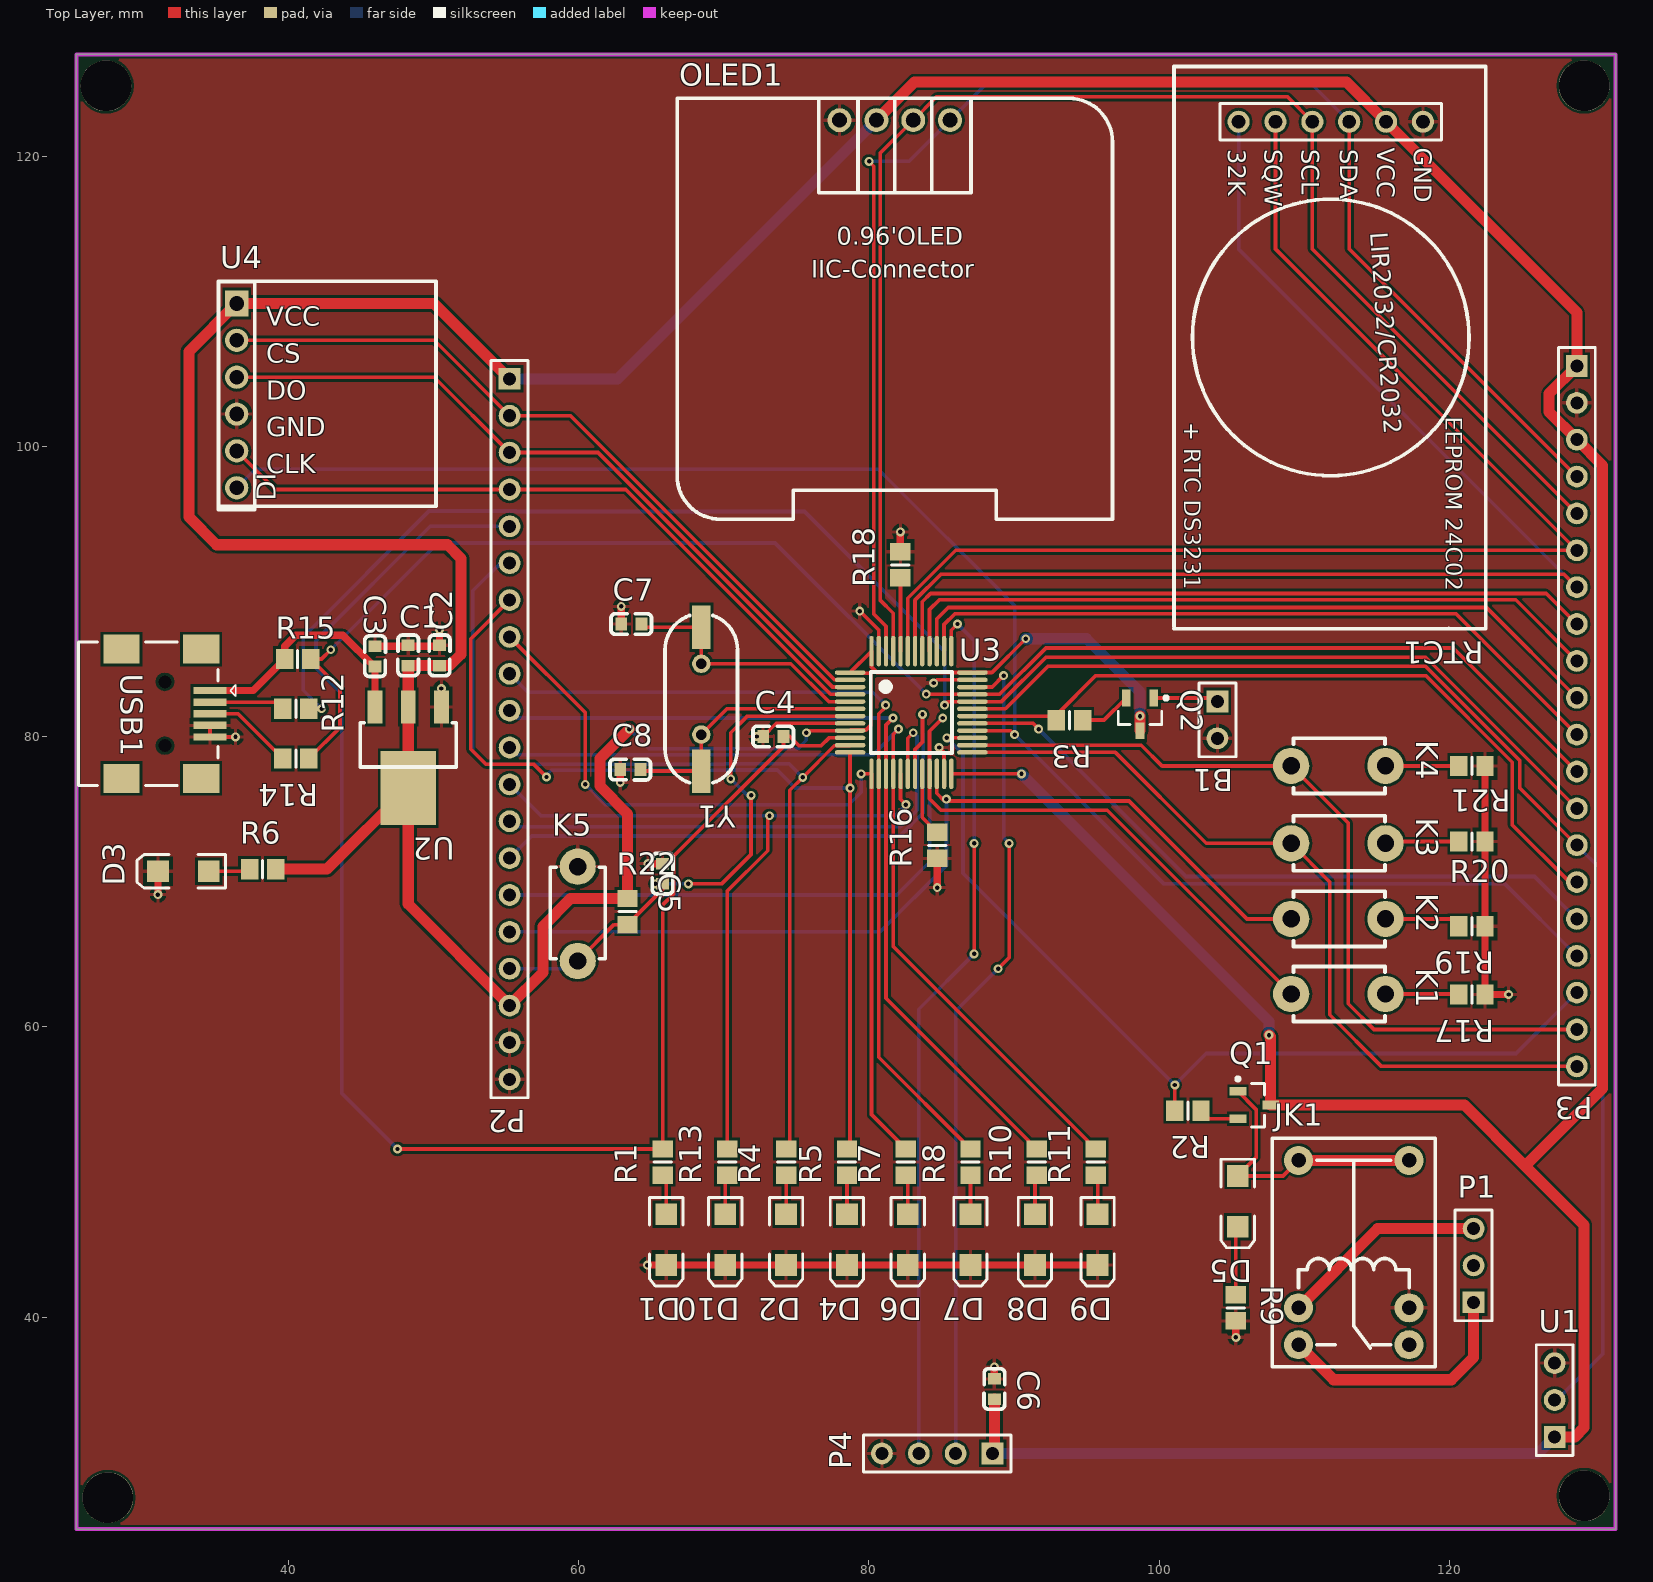
[diagram p0: Top Layer view]
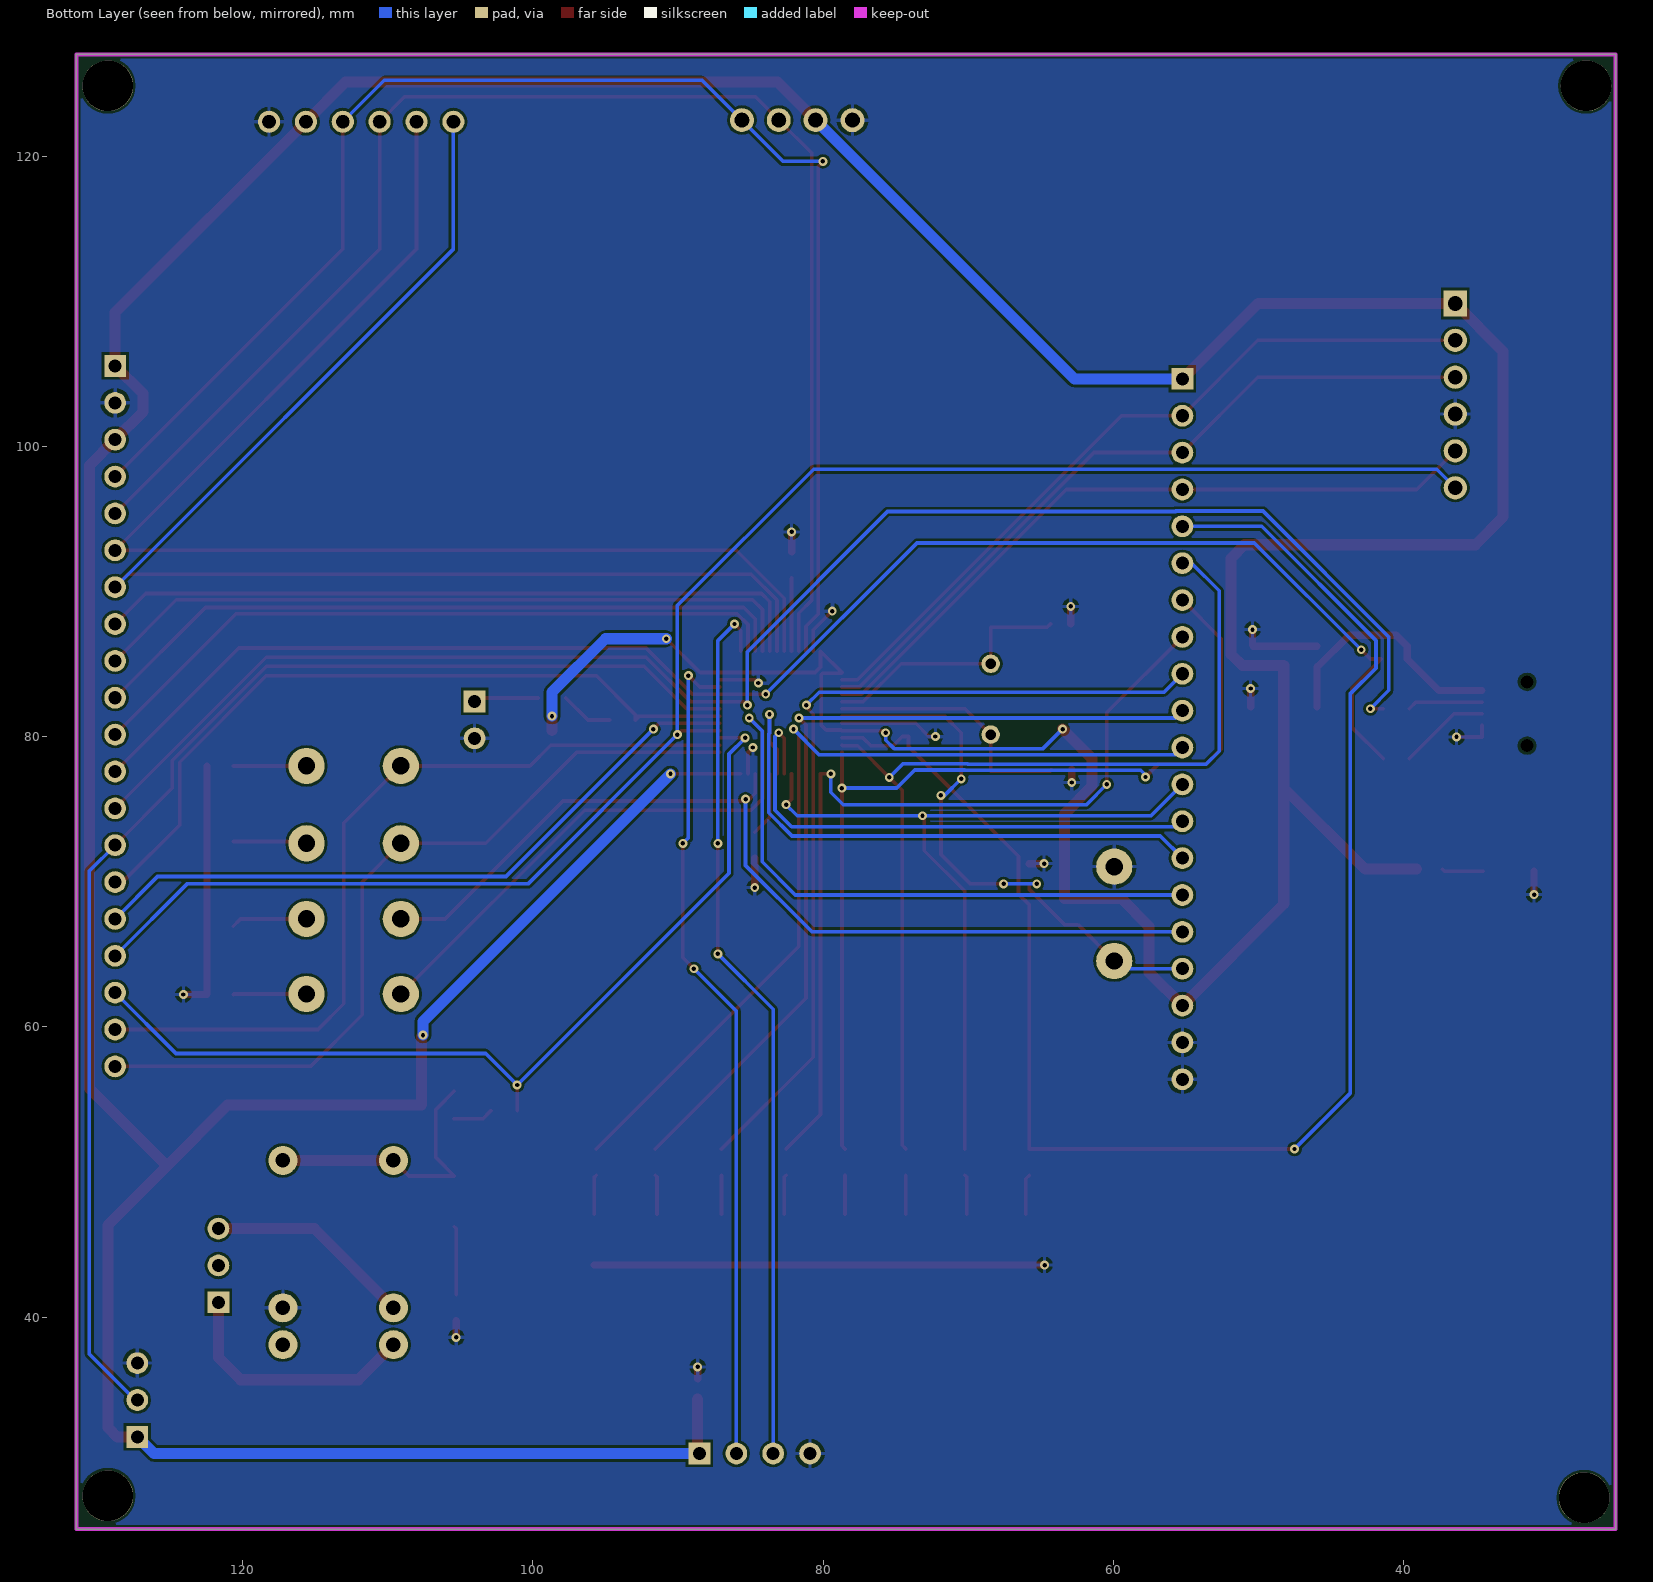
[diagram p1: Bottom Layer view, seen from below]
# Altium PCB MISC82098.PcbDoc
Units mm, origin at the board's own origin, x right, y up, seen from the top; angles counter-clockwise.
Board outline 106.05 x 101.6 mm, 2 copper layers (Top Layer, Bottom Layer); 61 components, 64 nets, 241 pads, 57 vias.

## Layer stack, top to bottom (the 12.6 mil dielectric is the usual default, probably not edited)
Top Solder: solder mask 0.0102, Solder Resist, Dk 3.5
Top Layer: signal copper 0.0356
Dielectric 1: dielectric 0.32, FR-4, Dk 4.8
Bottom Layer: signal copper 0.0356
Bottom Solder: solder mask 0.0102, Solder Resist, Dk 3.5

## Board outline
25.4,25.4 25.4,127 131.445,127 131.445,25.4

## Design rules (kind name [scope] priority, off if disabled: settings)
Clearance [All] p1: gap=0.178
MinimumSolderMaskSliver [All] p1: minsoldermaskwidth=0
PolygonConnect [All] p1: connectstyle=Relief reliefconductorwidth=0.254 reliefentries=4 polygonreliefangle="90 Angle" airgapwidth=0.254
RoutingVias [All] p1: holewidth=0.711 width=1.27 viastyle="Through Hole" minholewidth=0.711 minwidth=1.27 maxholewidth=0.711 maxwidth=1.27
SilkToSilkClearance [All] p1: silktosilkclearance=0
SilkToSolderMaskClearance [IsPad] p1: minsilkscreentomaskgap=0 clearancetoexposedcopper=TRUE
SolderMaskExpansion [All] p1: expansion=0.102
Width [All] p1: maxlimit=0.762 minlimit=0.254 preferedwidth=0.254
27 further rules are at their usual default settings.

## Components (designator, comment, footprint, x,y, rotation, side; value= is the part's Value field where it differs from the comment)
B1 "BEEP" HDR1X2 104.013,82.423 r270 top
C1 "10uF" C0603 48.26,85.598 r270 top
C2 "0.1uF" C0603 50.419,85.598 r270 top
C3 "10uF" C0603 45.977,85.541 r270 top
C4 "0.1uF" C0603 73.406,80.01 r0 top
C5 "0.1uF" C0603 65.789,70.558 r270 top
C6 "100NF" C0603 88.646,35.052 r270 top
C7 "20pF" C0603 63.627,87.757 r0 top
C8 "20pF" C0603 63.557,77.727 r0 top
D1 "POWER" 3.2X1.6X1.1 66.04,45.339 r270 top
D2 "POWER" 3.2X1.6X1.1 74.295,45.339 r270 top
D3 "POWER" 3.2X1.6X1.1 32.764,70.719 r180 top
D4 "POWER" 3.2X1.6X1.1 78.486,45.339 r270 top
D5 "POWER" 3.2X1.6X1.1 105.41,47.978 r270 top
D6 "POWER" 3.2X1.6X1.1 82.677,45.339 r270 top
D7 "POWER" 3.2X1.6X1.1 86.995,45.339 r270 top
D8 "POWER" 3.2X1.6X1.1 91.44,45.339 r270 top
D9 "POWER" 3.2X1.6X1.1 95.758,45.339 r270 top
D10 "POWER" 3.2X1.6X1.1 70.104,45.339 r270 top
JK1 "HK4100F-DC5V-SHG" HK4100F 113.411,44.45 r90 top
K1 "KEY" DIP-3X6X4.3 109.093,62.265 r0 top
K2 "KEY" DIP-3X6X4.3 109.093,67.437 r0 top
K3 "KEY" DIP-3X6X4.3 109.093,72.649 r0 top
K4 "KEY" DIP-3X6X4.3 109.093,77.978 r0 top
K5 "KEY" DIP-3X6X4.3 59.939,64.538 r90 top
OLED1 "0.96OLED_4P_MODULE_JX" 0.96OLED_4P 81.788,109.474 r0 top
P1 "Header 3" HDR1X3 121.666,41.021 r90 top
P2 "Header 20" HDR1X20 55.245,104.648 r270 top
P3 "Header 20" HDR1X20 128.778,105.537 r270 top
P4 "Header 4" HDR1X4 88.519,30.607 r180 top
Q1 "PNP" SOT-23B_N 106.553,54.61 r0 top
Q2 "PNP" SOT-23B_N 98.679,81.534 r270 top
R1 "330" 6-0805_N 65.786,50.684 r90 top
R2 "1K" 6-0805_N 101.981,54.229 r180 top
R3 "4.7K" 6-0805_N 93.822,81.137 r180 top
R4 "330" 6-0805_N 74.295,50.684 r90 top
R5 "330" 6-0805_N 78.486,50.684 r90 top
R6 "330" 6-0805_N 38.227,70.866 r0 top
R7 "330" 6-0805_N 82.55,50.684 r90 top
R8 "330" 6-0805_N 86.995,50.684 r90 top
R9 "1K" 6-0805_N 105.283,40.64 r270 top
R10 "330" 6-0805_N 91.567,50.684 r90 top
R11 "330" 6-0805_N 95.631,50.684 r90 top
R12 "100" 6-0805_N 40.513,81.915 r180 top
R13 "330" 6-0805_N 70.231,50.684 r90 top
R14 "100" 6-0805_N 40.513,78.486 r180 top
R15 "10K" 6-0805_N 40.64,85.344 r180 top
R16 "10K" 6-0805_N 84.709,72.506 r90 top
R17 "10K" 6-0805_N 121.55,62.23 r180 top
R18 "10K" 6-0805_N 82.169,91.832 r90 top
R19 "10K" 6-0805_N 121.55,66.929 r180 top
R20 "10K" 6-0805_N 121.55,72.771 r180 top
R21 "10K" 6-0805_N 121.55,77.978 r180 top
R22 "10K" 6-0805_N 63.373,67.945 r90 top
RTC1 "DS3231-RTC-SINGLE-HEADER" DS3231-RTC-24C32-EEPROM-SINGLE-HEADER 111.76,106.807 r270 top
U1 "DHT11" HDR1X3 127.254,31.75 r90 top
U2 "AMS1117" SOT223 48.26,82.042 r180 top
U3 "STM32F103C8T6" "LQFP48 7X7" 82.931,81.661 r270 top
U4 "W25Q128  SPI-Flash外部存储器" "SPI FLASH" 42.672,103.505 r0 top
USB1 "MINI-USB" USB-MINI-A 34.604,83.175 r270 top
Y1 "12M" XTAL_US 68.453,85.017 r270 top

## Footprints (in the part's own frame and the unit in brackets; to place one, negate y for a bottom-side part, rotate by r counter-clockwise, add the part's x,y. Pads: shape width x height; smd on the part's side, far side on the other; paste and mask are expansions set on the pad)
0.96OLED_4P [mm]
  round 1.65 hole 1 slot 1.005 at 0 deg paste+0 mask+0.051: 1(-3.811,12.997) 2(-1.271,13) 3(1.269,13) 4(3.809,13)
  silkscreen extent -15,-14.5 15,14.5
3.2X1.6X1.1 [mm] "SMT LED; 2 Flat Leads"
  rect 1.5x1.5 smd: 1(-1.75,0) 2(1.75,0)
  silkscreen extent -2.9,-1.15 3.2,1.15
6-0805_N [mm] "Chip Resistor, Body 2.0x1.2mm, IPC Medium Density"
  rect 1.2x1.4 smd: 1(-0.9,0) 2(0.9,0)
  silkscreen extent 0,-0.6 0,0.6, body extent -1.07,-0.7 1.07,0.7, height 0.7
C0603 [mm]
  rect 0.8x0.9 smd paste+0 mask+0.051: 1(-0.692,-0.003) 2(0.708,-0.003)
  silkscreen extent -1.4,-0.71 1.4,0.71
DIP-3X6X4.3 [mm]
  round 2.5 hole 1.2: 1(0,0) 3(6.5,0)
  silkscreen extent 0.16,-1.9 6.46,1.9, body extent -0.64,-1.75 7.19,1.75, height 4.31
DS3231-RTC-24C32-EEPROM-SINGLE-HEADER [mil]
  round 60 hole 36 slot 36.2 at 90 deg paste+0 mask+2: 1(-612.5,-247.5) 2(-612.5,-147.5) 3(-612.5,-47.5) 4(-612.5,52.5) 5(-612.5,152.5) 6(-612.5,252.5)
  silkscreen extent -763,-423 763,423
HDR1X2 [mm] "Connector; Header; 2 Position"
  rect 1.5x1.5 hole 0.9: 1(0,0)
  round 1.5 hole 0.9: 2(2.54,0)
  silkscreen extent -1.27,-1.27 3.81,1.27
HDR1X3 [mm] "Connector; Header; 3 Position"
  rect 1.5x1.5 hole 0.9: 1(0,0)
  round 1.5 hole 0.9: 2(2.54,0) 3(5.08,0)
  silkscreen extent -1.27,-1.27 6.35,1.27
HDR1X4 [mm] "Connector; Header; 4 Position"
  rect 1.5x1.5 hole 0.9: 1(0,0)
  round 1.5 hole 0.9: 2(2.54,0) 3(5.08,0) 4(7.62,0)
  silkscreen extent -1.27,-1.27 8.89,1.27
HDR1X20 [mm] "Connector; Header; 20 Position"
  rect 1.5x1.5 hole 0.9: 1(0,0)
  round 1.5 hole 0.9: 2(2.54,0) 3(5.08,0) 4(7.62,0) 5(10.16,0) 6(12.7,0) 7(15.24,0) 8(17.78,0) 9(20.32,0) 10(22.86,0) 11(25.4,0) 12(27.94,0) 13(30.48,0) 14(33.02,0) 15(35.56,0) 16(38.1,0) 17(40.64,0) 18(43.18,0) 19(45.72,0) 20(48.26,0)
  silkscreen extent -1.27,-1.27 49.53,1.27
HK4100F [mm] "单刀双投"
  round 2 hole 1: 1(-3.81,3.81) 2(-3.81,-3.81) 3(6.35,-3.81) 3(6.35,3.81) 4(-6.35,3.81) 5(-6.35,-3.81)
  silkscreen extent -7.87,-5.61 7.87,5.61, body extent -7.75,-5.5 7.75,5.5, height 12.2
"LQFP48 7X7" [mm]
  oval 0.3x2.1 smd: 1(-2.75,-4.227) 2(-2.25,-4.227) 3(-1.75,-4.227) 4(-1.25,-4.227) 5(-0.75,-4.227) 6(-0.25,-4.227) 7(0.25,-4.227) 8(0.75,-4.227) 9(1.25,-4.227) 10(1.75,-4.227) 11(2.25,-4.227) 12(2.75,-4.227) 25(2.75,4.202) 26(2.25,4.202) 27(1.75,4.202) 28(1.25,4.202) 29(0.75,4.202) 30(0.25,4.202) 31(-0.25,4.202) 32(-0.75,4.202) 33(-1.25,4.202) 34(-1.75,4.202) 35(-2.25,4.202) 36(-2.75,4.202)
  oval 2.1x0.3 smd: 13(4.227,-2.75) 14(4.227,-2.25) 15(4.227,-1.75) 16(4.227,-1.25) 17(4.227,-0.75) 18(4.227,-0.25) 19(4.227,0.25) 20(4.227,0.75) 21(4.227,1.25) 22(4.227,1.75) 23(4.227,2.25) 24(4.227,2.75) 37(-4.227,2.75) 38(-4.227,2.25) 39(-4.227,1.75) 40(-4.227,1.25) 41(-4.227,0.75) 42(-4.227,0.25) 43(-4.227,-0.25) 44(-4.227,-0.75) 45(-4.227,-1.25) 46(-4.227,-1.75) 47(-4.227,-2.25) 48(-4.227,-2.75)
  silkscreen extent -2.79,-2.79 2.79,2.79, body extent -4.51,-4.5 4.5,4.5, height 1.45
SOT223 [mil]
  rect 40x90 smd: 1(-90,0) 2(0,0) 3(90,0)
  rect 150x200 smd: 2(0,220)
  silkscreen extent -130,43 130,163, body extent -130,-30 126,246, height 65
SOT-23B_N [mm] "SOT23, 3-Leads, Body 2.9x1.3mm, Pitch 0.95mm, Lead Span 2.4mm, IPC Medium Density"
  rect 1.15x0.6 smd: 1(-1.125,0.95) 2(-1.125,-0.95) 3(1.125,0)
  silkscreen extent -1.25,-1.5 0.7,1.92, body extent -0.7,-1.5 0.7,1.5, height 1.14
"SPI FLASH" [mm]
  rect 1.6x1.8 hole 1.02 paste+0 mask+0.051: 1(-6.23,6.338)
  round 1.6 hole 1.02 paste+0 mask+0.051: 2(-6.23,3.798) 3(-6.23,1.258) 4(-6.23,-1.282) 5(-6.23,-3.822) 6(-6.23,-6.362)
  silkscreen extent -7.5,-7.86 7.5,7.86
USB-MINI-A [mm]
  rect 2x2.5 smd: 0(-2.85,-0.608) 0(-2.85,-6.108) 0(6.05,-0.608) 0(6.05,-6.108)
  rect 0.5x2.3 smd: 1(0,0) 2(0.8,0) 3(1.6,0) 4(2.4,0) 5(3.2,0)
  round 0.6 hole 0.9 unplated: MH1(3.8,-3.108) MH2(-0.6,-3.108)
  silkscreen extent -3.35,-9.06 6.55,1.78, body extent -3.17,-9.04 6.33,0.66, height 3.95
XTAL_US [mm]
  rect 3x1.27 smd: 1(-2.51,0) 2(7.39,0)
  round 1.27 hole 0.711: 1(0,0) 2(4.88,0)
  silkscreen extent -3.33,-2.5 8.21,2.5

## Part data
B1: "buzzer"
C1 C2 C3 C4 C5 C6 C7 C8: library part CAP, "non-polarized capacitor"
D1 D2 D3 D4 D5 D6 D7 D8 D9 D10: library part LED2, "Typical RED, GREEN, YELLOW, AMBER GaAs LED"
JK1: library part HK4100F, "changeover switch set"
P1: "Header, 3-Pin"
P2 P3: "Header, 20-Pin"
P4: "Header, 4-Pin"
Q1 Q2: "PNP Bipolar Transistor"
R1 R2 R3 R4 R5 R6 R7 R8 R9 R10 R11 R12 R13 R14 R15 R16 R17 R18 R19 R20 R21 R22: library part RES
U1: library part "Header 3", "Header, 3-Pin"
U2: "three-terminal voltage regulator"
Y1: library part XTAL, "Crystal Oscillator"

## Free pads (board coordinates)
  round 3.5 hole 3.5: 2(27.432,124.841) 3(27.559,27.559) 4(129.286,27.686) 5(129.286,124.841)

## Via types
v1: diameter 0.61, hole 0.305, Top Layer to Bottom Layer, 57 vias

## Nets (pads, with @x,y where several pads share a name; then routed paths per layer and width w, separated by ;. In a path a pad name is that pad's centre, name@x,y a point inside that pad or via, vN(x,y) a via of type N, cw(c..) or ccw(c..) an arc to the next point about the centre after c; other vN are vias at no path point)
3V3: C1.2 C2.2 C6.2 OLED1.2 P2.1 P2.18 P3.1 P3.3 P4.1 Q1.3 Q2.3 R6.2 R22.2 RTC1.5 U1.1 U2.2 U3.1 U3.9 U3.24 U3.36 U3.48 U4.1 | length 452.7
  Top Layer w0.254: v1(75.692,80.264) 75.692,80.304 75.799,80.411 U3.9 78.749,80.456 79.792,80.456 80.137,80.801 80.137,84.27 80.041,84.366 78.749,84.366 U3.1 U3.48 80.181,84.792 80.562,84.411 U3.36 88.475,84.411 v1(90.805,86.741) ; U3.24 v1(90.515,77.434)
  Top Layer w0.762: R6.2 42.672,70.866 U2.2@48.26,76.454 ; P2.1 50.05,109.843 U4.1 33.147,106.548 33.147,95.123 35.052,93.218 50.952,93.218 51.892,92.278 51.892,85.674 51.108,84.89 C2.2 C1.2 48.26,84.888 48.26,82.042 U2.2@48.26,76.454 ; v1(63.5,80.518) 61.468,78.486 61.468,76.581 63.373,74.676 R22.2 59.447,68.845 57.531,66.929 57.531,63.754 P2.18 48.26,68.453 U2.2@48.26,76.454 ; OLED1.2 83.138,125.095 112.903,125.095 RTC1.5 128.778,109.22 P3.1 126.873,103.632 126.873,102.362 P3.3 130.556,98.679 130.556,55.753 125.222,50.419 ; P4.1 88.643,30.731 C6.2 ; Q2.3 v1(98.679,81.407) ; v1(107.569,59.436) 107.678,59.327 Q1.3 121.031,54.61 125.222,50.419 ; U1.1 128.651,31.75 129.286,32.385 129.286,46.355 125.222,50.419
  Bottom Layer w0.254: v1(63.5,80.518) 64.846,79.172 75.108,79.172 75.692,79.756 v1(75.692,80.264)
  Bottom Layer w0.762: P2.1 62.691,104.648 OLED1.2 ; P4.1 126.111,30.607 U1.1 ; v1(90.515,77.434) 107.569,60.38 v1(107.569,59.436) ; v1(90.805,86.741) 94.996,86.741 98.679,83.058 v1(98.679,81.407)
+5: C3.2 R15.2 U2.3 USB1.1 | length 17.2
  Top Layer w0.508: USB1.1 37.571,83.175 R15.2 39.74,86.222 40.513,86.995 43.751,86.995 45.913,84.833 C3.2 U2.3
BOOT: R18.1 U3.44 | length 5
  Top Layer w0.254: R18.1 82.181,90.92 U3.44
GND: B1.2 C1.1 C2.1 C3.1 C4.1 C5.1 C6.1 C7.1 C8.1 D1.2 D2.2 D3.2 D4.2 D6.2 D7.2 D8.2 D9.2 D10.2 JK1.2 K5.3 OLED1.1 P2.19 P2.20 P3.2 P4.4 R9.2 R16.1 R17.1 R18.2 R19.1 R20.1 R21.1 RTC1.6 U1.3 U2.1 U3.8 U3.23 U3.35 U3.47 U4.4 USB1.4 USB1.5 | length 82.4
  Top Layer w0.254: USB1.4 USB1.5 v1(36.357,79.975) ; v1(72.266,80.007) C4.1 73.618,80.911 U3.8 ; v1(79.375,88.646) 80.681,87.34 U3.47 ; v1(84.455,83.693) 84.673,83.911 U3.35 ; v1(84.836,79.248) 85.181,78.903 U3.23
  Top Layer w0.508: v1(31.014,69.114) D3.2 ; C3.1 50.359,86.233 C2.1 v1(50.416,87.373) ; U2.1 v1(50.546,83.312) ; v1@62.865,77.089 C8.1 ; C7.1 v1(62.935,88.97) ; v1(64.742,43.589) D1.2 D10.2 D2.2 D4.2 D6.2 D7.2 D8.2 D9.2 ; v1(64.773,71.25) C5.1 ; R18.2 v1(82.169,94.107) ; v1(84.709,69.596) R16.1 ; C6.1 v1(88.643,36.573) ; v1(105.283,38.608) R9.2 ; R21.1 R20.1 R19.1 R17.1 v1(124.079,62.23)
  other v1: 62.865,76.835
K1: K1.1 P2.15 U3.21 | length 76.6
  Top Layer w0.254: v1(85.09,81.28) 84.181,80.371 U3.21 84.181,75.712 84.963,74.93 96.428,74.93 K1.1
  Bottom Layer w0.254: P2.15 81.915,69.088 84.201,71.374 84.201,80.391 v1(85.09,81.28)
K2: K2.1 P2.16 U3.22 | length 65.9
  Top Layer w0.254: U3.22 84.681,76.101 85.217,75.565 97.917,75.565 106.045,67.437 K2.1
  Bottom Layer w0.254: P2.16 80.772,66.548 85.344,71.12 v1(85.344,75.692)
K3: K3.1 P3.20 U3.25 | length 56
  Top Layer w0.254: U3.25 96.984,78.911 103.246,72.649 K3.1 111.76,69.982 111.76,60.833 115.316,57.277 P3.20
K4: K4.1 P3.19 U3.26 | length 57.1
  Top Layer w0.254: U3.26 98.77,79.411 100.203,77.978 K4.1 113.03,74.041 113.03,61.595 114.808,59.817 P3.19
NetB1_1: B1.1 Q2.1 | length 4.5
  Top Layer w0.254: Q2.1 103.777,82.659 B1.1
NetD1_1: D1.1 R1.1 | length 2.8
  Top Layer w0.254: R1.1 66.04,49.53 D1.1
NetD2_1: D2.1 R4.1 | length 2.7
  Top Layer w0.254: D2.1 R4.1
NetD3_1: D3.1 R6.1 | length 2.9
  Top Layer w0.254: D3.1 37.18,70.719 R6.1
NetD4_1: D4.1 R5.1 | length 2.7
  Top Layer w0.254: D4.1 R5.1
NetD5_1: D5.1 JK1.3 Q1.1 | length 19.1
  Top Layer w0.254: Q1.1 106.68,54.308 106.68,50.998 D5.1 108.529,49.728 JK1.3@109.601,50.8
  Top Layer w0.762: JK1.3@109.601,50.8 JK1.3@117.221,50.8
NetD5_2: D5.2 R9.1 | length 4.7
  Top Layer w0.254: R9.1 105.283,46.101 D5.2
NetD6_1: D6.1 R7.1 | length 2.7
  Top Layer w0.254: R7.1 82.677,49.657 D6.1
NetD7_1: D7.1 R8.1 | length 2.7
  Top Layer w0.254: D7.1 R8.1
NetD8_1: D8.1 R10.1 | length 2.7
  Top Layer w0.254: D8.1 91.44,49.657 R10.1
NetD9_1: D9.1 R11.1 | length 2.7
  Top Layer w0.254: R11.1 95.758,49.657 D9.1
NetD10_1: D10.1 R13.1 | length 2.7
  Top Layer w0.254: D10.1 70.104,49.657 R13.1
NetJK1_1: JK1.1 P1.3 | length 14.3
  Top Layer w0.762: JK1.1 115.062,46.101 P1.3
NetJK1_4: JK1.4 P1.1 | length 17.5
  Top Layer w0.762: JK1.4 112.014,35.687 120.142,35.687 121.666,37.211 P1.1
NetK1_3: K1.3 R17.2 | length 5.1
  Top Layer w0.254: K1.3 120.615,62.265 R17.2
NetK2_3: K2.3 R19.2 | length 5.3
  Top Layer w0.254: K2.3 120.142,67.437 R19.2
NetK3_3: K3.3 R20.2 | length 5.1
  Top Layer w0.254: K3.3 115.715,72.771 R20.2
NetK4_3: K4.3 R21.2 | length 5.1
  Top Layer w0.254: K4.3 R21.2
NetQ1_2: Q1.2 R2.1 | length 2.8
  Top Layer w0.254: R2.1 103.45,53.66 Q1.2
NetQ2_2: Q2.2 R3.1 | length 3.6
  Top Layer w0.254: R3.1 96.207,81.137 Q2.2
NetR12_2: R12.2 USB1.2 | length 5.2
  Top Layer w0.254: USB1.2 39.153,82.375 R12.2
NetR14_2: R14.2 USB1.3 | length 6.3
  Top Layer w0.254: USB1.3 36.524,81.575 R14.2
NRST: C5.2 K5.1 P2.17 R22.1 U3.7 | length 38.4
  Top Layer w0.254: K5.1 62.446,67.045 R22.1 65.786,69.458 C5.2 ; v1(67.564,69.85) 69.85,69.85 71.882,71.882 v1(71.882,75.946) ; v1(70.485,77.089) 70.485,80.264 71.632,81.411 U3.7
  Bottom Layer w0.254: P2.17 59.409,64.008 K5.1 ; v1(65.278,69.85) v1(67.564,69.85) ; v1(70.485,77.089) 71.628,75.946 v1(71.882,75.946)
OSC_IN: C7.2 U3.5 Y1.1 | length 18.1
  Top Layer w0.254: C7.2 64.562,87.527 68.453,87.527 68.453,85.017 74.622,85.017 77.228,82.411 U3.5
OSC_OUT: C8.2 U3.6 Y1.2 | length 17.7
  Top Layer w0.254: C8.2 64.362,77.627 68.453,77.627 68.453,80.137 70.227,81.911 U3.6
PA0: C4.2 P2.5 R1.2 U3.10 | length 109.2
  Top Layer w0.254: v1(47.52,51.584) R1.2 65.786,68.39 66.541,69.145 66.541,71.748 74.114,79.321 C4.2 74.552,80.007 75.184,79.375 76.708,79.375 77.244,79.911 U3.10
  Bottom Layer w0.254: v1(47.52,51.584) 43.688,55.416 43.688,82.931 41.91,84.709 41.91,86.614 49.784,94.488 P2.5
PA1: P2.6 R4.2 U3.11 | length 68.1
  Top Layer w0.254: R4.2 74.549,51.838 74.549,76.299 v1(75.438,77.188) 77.616,79.366 78.659,79.366 U3.11
  Bottom Layer w0.254: P2.6 54.61,91.948 52.705,90.043 52.705,78.994 53.594,78.105 70.028,78.105 70.054,78.13 74.496,78.13 v1(75.438,77.188)
PA2: P2.7 R5.2 U3.12 | length 66.5
  Top Layer w0.254: P2.7 52.578,86.741 52.578,79.121 53.594,78.105 56.896,78.105 v1(57.785,77.216) ; R5.2 78.704,51.802 v1(78.704,76.454) U3.12
  Bottom Layer w0.254: v1(57.785,77.216) 57.785,77.343 58.115,77.673 70.207,77.673 70.232,77.699 73.685,77.699 74.93,76.454 v1(78.704,76.454)
PA3: P2.8 R7.2 U3.13 | length 61.1
  Top Layer w0.254: P2.8 60.452,81.661 v1(60.452,76.708) ; v1(79.466,77.434) U3.13 80.181,53.953 R7.2
  Bottom Layer w0.254: v1(60.452,76.708) 61.849,75.311 78.613,75.311 79.466,76.164 v1(79.466,77.434)
PA4: P2.9 R8.2 U3.14 | length 60.2
  Top Layer w0.254: v1(81.153,82.169) 81.153,82.042 80.681,81.57 U3.14 80.681,57.898 R8.2
  Bottom Layer w0.254: P2.9 56.515,83.058 80.264,83.058 v1(81.153,82.169)
PA5: P2.10 R10.2 U3.15 | length 60.8
  Top Layer w0.254: v1(81.661,81.28) 81.181,80.8 U3.15 81.181,61.97 R10.2
  Bottom Layer w0.254: P2.10 55.753,81.28 v1(81.661,81.28)
PA6: P2.11 R11.2 U3.16 | length 62.6
  Top Layer w0.254: v1(82.042,80.518) 81.681,80.157 U3.16 81.681,65.534 R11.2
  Bottom Layer w0.254: P2.11 55.753,78.74 80.264,78.74 v1(82.042,80.518)
PA7: P2.12 R13.2 U3.17 | length 55
  Top Layer w0.254: R13.2 70.231,69.342 73.025,72.136 73.025,74.422 v1(73.152,74.549) ; U3.17 82.181,75.68 v1(82.55,75.311)
  Bottom Layer w0.254: P2.12 57.404,74.549 v1(73.152,74.549) 81.788,74.549 v1(82.55,75.311)
PA8: P3.16 U3.29 | length 47.2
  Top Layer w0.254: U3.29 91.301,80.911 v1(91.694,80.518)
  Bottom Layer w0.254: v1(91.694,80.518) 101.854,70.358 125.857,70.358 P3.16
PA9: P3.15 R3.2 U3.30 | length 51.7
  Top Layer w0.254: U3.30 92.648,81.411 R3.2 92.922,81.492 95.631,84.201 118.364,84.201 124.333,78.232 124.333,73.914 128.27,69.977 P3.15
PA10: P3.14 U1.2 U3.31 | length 90.1
  Top Layer w0.254: U3.31 89.404,81.911 92.329,84.836 118.364,84.836 124.841,78.359 124.841,76.454 P3.14
  Bottom Layer w0.254: U1.2@126.873,33.782 130.556,37.465 130.556,70.739 P3.14
PA11: P3.13 R12.1 U3.32 | length 111.1
  Top Layer w0.254: R12.1 v1(42.291,81.915) ; v1(85.217,82.169) 85.459,82.411 U3.32 89.142,82.411 92.202,85.471 118.364,85.471 P3.13
  Bottom Layer w0.254: v1(42.291,81.915) 41.021,83.185 41.021,86.868 49.696,95.543 55.682,95.543 55.721,95.504 75.565,95.504 85.217,85.852 v1(85.217,82.169)
PA12: P3.12 R14.1 R15.1 U3.33 | length 108.3
  Top Layer w0.254: R14.1 43.561,80.634 43.561,83.323 R15.1 42.291,85.344 v1(42.926,85.979) ; v1(83.947,82.931) 83.967,82.911 U3.33 89.007,82.911 92.202,86.106 120.269,86.106 P3.12
  Bottom Layer w0.254: v1(42.926,85.979) 50.292,93.345 73.533,93.345 v1(83.947,82.931)
PA13: P4.2 U3.34 | length 57.8
  Top Layer w0.254: U3.34 88.491,83.411 v1(89.281,84.201) ; v1(88.9,64.008) 89.662,64.77 v1(89.662,72.644)
  Bottom Layer w0.254: P4.2 85.979,61.087 v1(88.9,64.008) ; v1(89.281,84.201) 89.281,73.025 v1(89.662,72.644)
PA14: P4.3 U3.37 | length 61.2
  Top Layer w0.254: U3.37 85.681,87.332 v1(86.106,87.757) ; v1(87.249,65.024) v1(87.249,72.644)
  Bottom Layer w0.254: P4.3 83.439,61.214 v1(87.249,65.024) ; v1(86.106,87.757) 87.249,86.614 v1(87.249,72.644)
PA15: P3.11 U3.38 | length 49.2
  Top Layer w0.254: U3.38 85.181,87.721 85.928,88.468 120.447,88.468 P3.11
PB0: P2.13 U3.18 | length 37.1
  Top Layer w0.254: U3.18 82.681,79.887 v1(83.058,80.264)
  Bottom Layer w0.254: P2.13 55.626,73.787 82.169,73.787 83.312,74.93 83.312,80.01 v1(83.058,80.264)
PB1: P2.14 U3.19 | length 40.8
  Top Layer w0.254: U3.19 83.181,79.117 83.693,79.629 v1(83.693,81.534)
  Bottom Layer w0.254: P2.14 56.769,73.152 82.145,73.152 83.744,74.751 83.744,80.189 83.693,80.24 v1@83.693,81.407
PB2: R16.2 U3.20 | length 4.5
  Top Layer w0.254: U3.20 83.681,74.434 R16.2
PB3: P3.10 U3.39 | length 49.2
  Top Layer w0.254: U3.39 84.681,88.11 85.471,88.9 122.555,88.9 P3.10
PB4: P3.9 U3.40 | length 49.5
  Top Layer w0.254: U3.40 84.181,88.753 84.861,89.433 124.562,89.433 P3.9
PB5: P3.8 U3.41 | length 49.6
  Top Layer w0.254: U3.41 83.681,89.293 84.253,89.865 126.67,89.865 P3.8
PB6: P3.7 RTC1.1 U3.42 | length 91.9
  Top Layer w0.254: U3.42 83.181,89.404 84.963,91.186 127.889,91.186 P3.7
  Bottom Layer w0.254: RTC1.1 105.474,113.602 P3.7
PB7: P3.6 RTC1.2 U3.43 | length 89.2
  Top Layer w0.254: U3.43 82.681,89.539 85.979,92.837 P3.6 108.013,113.602 RTC1.2
PB8: OLED1.3 P3.5 RTC1.3 U3.45 | length 101.3
  Top Layer w0.254: U3.45 81.681,88.499 80.772,89.408 80.772,120.189 OLED1.3 84.662,124.079 108.839,124.079 RTC1.3 110.553,113.602 P3.5
PB9: OLED1.4 P3.4 RTC1.4 U3.46 | length 101.8
  Top Layer w0.254: v1(80.01,119.634) 80.34,119.304 80.34,88.443 81.181,87.602 U3.46 ; RTC1.4 113.093,113.602 P3.4
  Bottom Layer w0.254: v1(80.01,119.634) 82.757,119.634 OLED1.4 88.345,125.222 110.236,125.222 RTC1.4
PB14: P3.18 R2.2 U3.27 | length 64.3
  Top Layer w0.254: v1(85.372,79.911) U3.27 ; R2.2 v1(101.081,55.996)
  Bottom Layer w0.254: v1(85.372,79.911) 86.487,78.796 86.487,70.59 v1(101.081,55.996) 103.251,58.166 124.587,58.166 P3.18
PB15: P3.17 U3.28 U4.6 | length 115
  Top Layer w0.254: U3.28 89.769,80.411 v1(90.043,80.137)
  Bottom Layer w0.254: U4.6 37.724,98.425 80.645,98.425 90.043,89.027 v1(90.043,80.137) 100.33,69.85 123.825,69.85 P3.17
PC13: P2.2 U3.2 U4.2 | length 52
  Top Layer w0.254: U4.2 50.05,107.303 P2.2 59.436,102.108 77.633,83.911 U3.2
PC14: P2.3 U3.3 U4.3 | length 51.1
  Top Layer w0.254: U4.3 50.05,104.763 P2.3 61.341,99.568 77.498,83.411 U3.3
PC15: P2.4 U3.4 U4.5 | length 49.2
  Top Layer w0.254: U4.5 39.097,97.028 P2.4 63.246,97.028 77.363,82.911 U3.4
pads on no net: JK1.5 P1.2 USB1.0 USB1.MH1 USB1.MH2

## Polygon pours and split planes (outlines as drawn)
GND on Top Layer "G" (solid, remove dead copper, pour order 4): 9.398,135.89 12.319,132.969 148.717,132.969 148.717,24.511 138.557,14.351 138.43,14.478 10.922,14.478
GND on Bottom Layer "G" (solid, remove dead copper, pour order 6): 23.241,17.907 141.097,17.907 145.034,21.844 145.542,22.352 145.542,136.398 17.653,136.398 14.478,133.223

## Keep-outs
Keep-Out Layer:
  the board outline again, w0.254